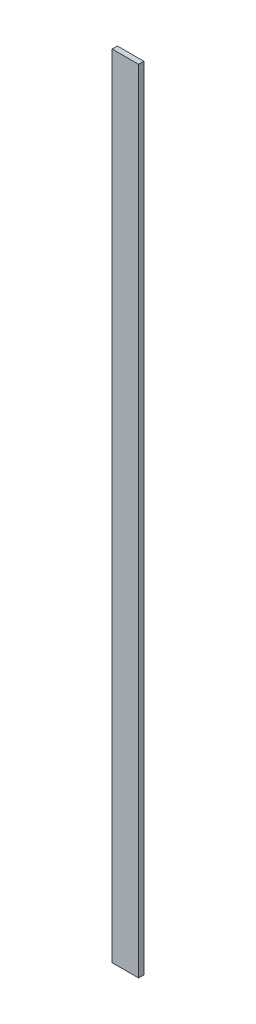
from build123d import *

# Parameters (mm, degrees)
SKETCH1_W           = 10
SKETCH1_H           = 300
BOSS_EXTRUDE1_DEPTH = 2


with BuildPart() as part:
    # Sketch1 → Boss-Extrude1 (new body)
    with BuildSketch(Plane.XY):
        with Locations((5, 150)):
            Rectangle(SKETCH1_W, SKETCH1_H)
    extrude(amount=BOSS_EXTRUDE1_DEPTH)


solid = part.part
